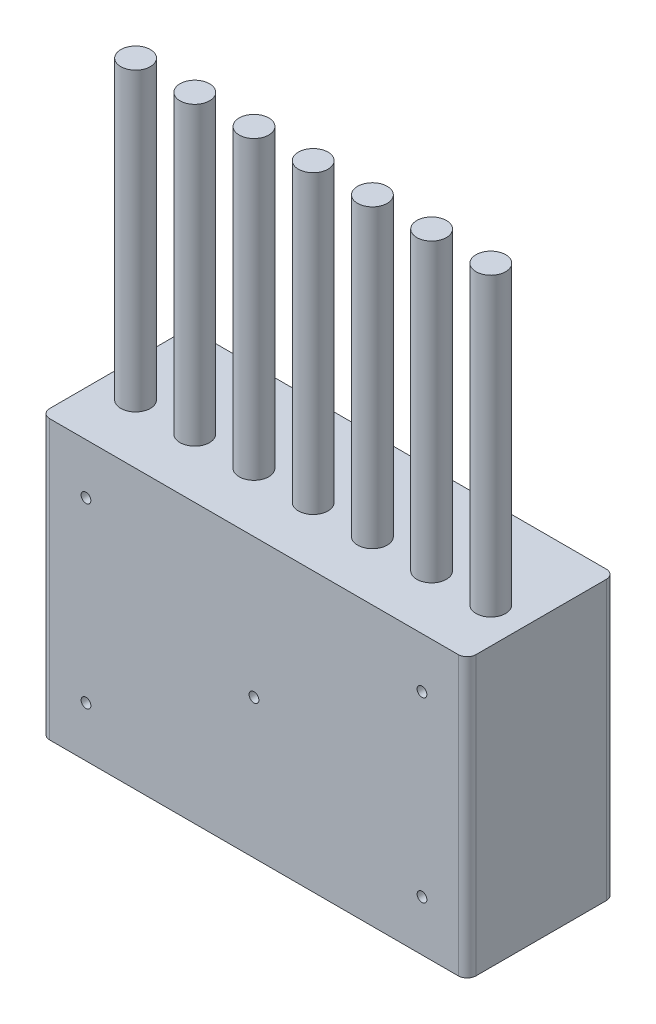
from build123d import *

# Parameters (mm, degrees)
SKETCH_1_W                  = 144
SKETCH_1_H                  = 94
EXTRUDE_1_DEPTH             = 50
SKETCH_2_R                  = 5
EXTRUDE_2_DEPTH             = 100
EXTRUDE_2_2_DEPTH           = 100
EXTRUDE_2_3_DEPTH           = 100
EXTRUDE_2_4_DEPTH           = 100
EXTRUDE_2_5_DEPTH           = 100
EXTRUDE_2_6_DEPTH           = 100
EXTRUDE_2_7_DEPTH           = 100
FILLET_1_R                  = 3
SKETCH_4_W                  = 1.65
SKETCH_4_H                  = 50
HOLE_WIZARD_M4_1_AT_2_COUNT = 2
HOLE_WIZARD_M4_1_AT_2_PITCH = 64.191607707
HOLE_WIZARD_M4_1_AT_3_COUNT = 2
HOLE_WIZARD_M4_1_AT_3_PITCH = 113.5
HOLE_WIZARD_M4_1_AT_4_COUNT = 2
HOLE_WIZARD_M4_1_AT_4_PITCH = 60
HOLE_WIZARD_M4_1_AT_5_COUNT = 2
HOLE_WIZARD_M4_1_AT_5_PITCH = 128.383215414


with BuildPart() as part:
    # 草图1 → 凸台-拉伸1 (new body)
    with BuildSketch(Plane.XY):
        Rectangle(SKETCH_1_W, SKETCH_1_H)
    extrude(amount=EXTRUDE_1_DEPTH)

    # 圆角1
    fillet_1_edges = [part.edges().sort_by_distance(p)[0] for p in [
        (-72, 0, 50),
        (72, 0, 50),
        (-72, 0, 0),
        (72, 0, 0),
    ]]
    fillet(fillet_1_edges, radius=FILLET_1_R)

    # 草图4 → M4 螺纹孔1 (revolve, cut)
    with BuildSketch(Plane(origin=(-56.75, 30, 50), x_dir=(0, -1, 0), z_dir=(1, 0, 0))):
        with Locations((0.825, 25)):
            Rectangle(SKETCH_4_W, SKETCH_4_H)
    hole_wizard_m4_1 = revolve(axis=Axis((-56.75, 30, 56.35), (0, 0, -1)), mode=Mode.SUBTRACT)

    # M4 螺纹孔1 at 2: M4 螺纹孔1 ×2
    with Locations(*[Vector(0.8840719531297252, -0.46735081222716746, 0) * (i * HOLE_WIZARD_M4_1_AT_2_PITCH) for i in range(1, HOLE_WIZARD_M4_1_AT_2_COUNT)]):
        add(hole_wizard_m4_1, mode=Mode.SUBTRACT)

    # M4 螺纹孔1 at 3: M4 螺纹孔1 ×2
    with Locations(*[(i * HOLE_WIZARD_M4_1_AT_3_PITCH, 0, 0) for i in range(1, HOLE_WIZARD_M4_1_AT_3_COUNT)]):
        add(hole_wizard_m4_1, mode=Mode.SUBTRACT)

    # M4 螺纹孔1 at 4: M4 螺纹孔1 ×2
    with Locations(*[(0, -i * HOLE_WIZARD_M4_1_AT_4_PITCH, 0) for i in range(1, HOLE_WIZARD_M4_1_AT_4_COUNT)]):
        add(hole_wizard_m4_1, mode=Mode.SUBTRACT)

    # M4 螺纹孔1 at 5: M4 螺纹孔1 ×2
    with Locations(*[Vector(0.8840719531297252, -0.46735081222716734, 0) * (i * HOLE_WIZARD_M4_1_AT_5_PITCH) for i in range(1, HOLE_WIZARD_M4_1_AT_5_COUNT)]):
        add(hole_wizard_m4_1, mode=Mode.SUBTRACT)


with BuildPart() as body_2:
    # 草图2 → 凸台-拉伸2 (new body)
    with BuildSketch(Plane(origin=(0, 47, 0), x_dir=(1, 0, 0), z_dir=(0, 1, 0))):
        with Locations(Location((0, -30, 0), (0, 0, 90))):
            Circle(SKETCH_2_R)
    extrude(amount=EXTRUDE_2_DEPTH)


with BuildPart() as body_3:
    # 草图2 → Extrude 2 2 (new body)
    with BuildSketch(Plane(origin=(0, 47, 0), x_dir=(1, 0, 0), z_dir=(0, 1, 0))):
        with Locations(Location((20, -30, 0), (0, 0, 90))):
            Circle(SKETCH_2_R)
    extrude(amount=EXTRUDE_2_2_DEPTH)


with BuildPart() as body_4:
    # 草图2 → Extrude 2 3 (new body)
    with BuildSketch(Plane(origin=(0, 47, 0), x_dir=(1, 0, 0), z_dir=(0, 1, 0))):
        with Locations(Location((40, -30, 0), (0, 0, 90))):
            Circle(SKETCH_2_R)
    extrude(amount=EXTRUDE_2_3_DEPTH)


with BuildPart() as body_5:
    # 草图2 → Extrude 2 4 (new body)
    with BuildSketch(Plane(origin=(0, 47, 0), x_dir=(1, 0, 0), z_dir=(0, 1, 0))):
        with Locations(Location((60, -30, 0), (0, 0, 90))):
            Circle(SKETCH_2_R)
    extrude(amount=EXTRUDE_2_4_DEPTH)


with BuildPart() as body_6:
    # 草图2 → Extrude 2 5 (new body)
    with BuildSketch(Plane(origin=(0, 47, 0), x_dir=(1, 0, 0), z_dir=(0, 1, 0))):
        with Locations(Location((-60, -30, 0), (0, 0, 90))):
            Circle(SKETCH_2_R)
    extrude(amount=EXTRUDE_2_5_DEPTH)


with BuildPart() as body_7:
    # 草图2 → Extrude 2 6 (new body)
    with BuildSketch(Plane(origin=(0, 47, 0), x_dir=(1, 0, 0), z_dir=(0, 1, 0))):
        with Locations(Location((-40, -30, 0), (0, 0, 90))):
            Circle(SKETCH_2_R)
    extrude(amount=EXTRUDE_2_6_DEPTH)


with BuildPart() as body_8:
    # 草图2 → Extrude 2 7 (new body)
    with BuildSketch(Plane(origin=(0, 47, 0), x_dir=(1, 0, 0), z_dir=(0, 1, 0))):
        with Locations(Location((-20, -30, 0), (0, 0, 90))):
            Circle(SKETCH_2_R)
    extrude(amount=EXTRUDE_2_7_DEPTH)


solid = Compound([part.part, body_2.part, body_3.part, body_4.part, body_5.part, body_6.part, body_7.part, body_8.part])
